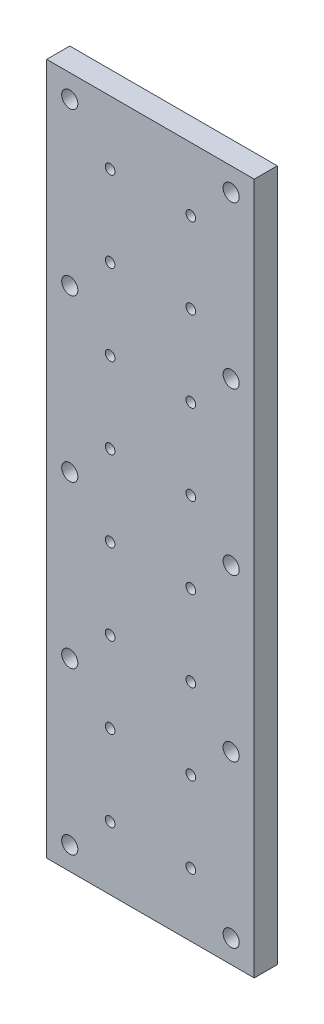
SolidWorks part; units mm, degrees
material "环氧酚醛层压布板3240"
ref_plane "Front Plane" through (0, 0, 0) normal (0, 0, 1) x (1, 0, 0)
ref_plane "Top Plane" through (0, 0, 0) normal (0, 1, 0) x (1, 0, 0)
ref_plane "Right Plane" through (0, 0, 0) normal (1, 0, 0) x (0, 0, -1)
other "Configuration Table"
sketch "Sketch1" plane through (0, 0, 0) normal (0, 0, 1) x (1, 0, 0)
  line L1 (-45, -150) -> (45, -150)
  line L2 (-45, -150) -> (-45, 150)
  line L3 (-45, 150) -> (45, 150)
  line L4 (45, -150) -> (45, 150)
  line L5 (-45, -150) -> (45, 150) construction
  line L6 (-45, 150) -> (45, -150) construction
  circle A0 centre (-35, 0) radius 5.5 construction
  point P0 (0, 0)
  dimension "D1" = 90
  dimension "D2" = 300
  dimension "D3" = 0
  dimension "D4" = 35
extrude "Boss-Extrude1" add sketch "Sketch1" along normal blind 10
hole_wizard "Ø7.0 (7) Diameter Hole1" positions "Sketch2" profile "Sketch4" hole size "Ø7.0" standard "GB" end condition through all
sketch "Sketch2" plane through (0, 0, 10) normal (0, 0, 1) x (1, 0, 0)
  point P0 (-35, 0)
sketch "Sketch4" plane through (-35, 0, 10) normal (1, 0, 0) x (0, -1, 0)
  line L0 (0, 0) -> (0, 10)
  line L1 (0, 10) -> (3.5, 10)
  line L2 (3.5, 10) -> (3.5, 0)
  line L5 (3.5, 0) -> (0, 0)
  line L11 (0, -6.35) -> (0, 107.95) construction
  dimension "通孔孔直径" = 7
  dimension "通孔孔深度" = 10
pattern_linear "LPattern1" count 3 spacing 70 along (0, -1, 0) count 2 spacing 70 along (1, 0, 0) of "Ø7.0 (7) Diameter Hole1"
pattern_linear "LPattern2" count 3 spacing 70 along (0, 1, 0) of "LPattern1", "Ø7.0 (7) Diameter Hole1"
sketch "Sketch5" plane through (0, 0, 0) normal (0, 0, -1) x (-1, 0, 0)
  line L0 (45, -150) -> (-45, 150) construction
  line L1 (-17.5, -17.5) -> (17.5, -17.5)
  line L2 (-17.5, -17.5) -> (-17.5, 17.5)
  line L3 (-17.5, 17.5) -> (17.5, 17.5)
  line L4 (17.5, -17.5) -> (17.5, 17.5)
  line L5 (-17.5, -17.5) -> (17.5, 17.5) construction
  line L6 (-17.5, 17.5) -> (17.5, -17.5) construction
  point P0 (0, 0)
  dimension "D1" = 35
  dimension "D2" = 35
hole_wizard "M5 Tapped Hole1" positions "Sketch6" profile "Sketch7" tap size "M5" standard "GB" end condition through all
sketch "Sketch6" plane through (0, 0, 0) normal (0, 0, -1) x (-1, 0, 0)
  point P0 (17.5, 17.5)
  point P3 (17.5, -17.5)
  point P6 (-17.5, -17.5)
  point P9 (-17.5, 17.5)
sketch "Sketch7" plane through (-17.5, 17.5, 0) normal (1, 0, 0) x (0, 1, 0)
  line L0 (0, 0) -> (0, 10)
  line L1 (0, 10) -> (2.1, 10)
  line L2 (2.1, 10) -> (2.1, 0)
  line L5 (2.1, 0) -> (0, 0)
  line L11 (0, -6.35) -> (0, 107.95) construction
  dimension "通孔螺纹孔钻头直径" = 4.2
  dimension "通孔螺纹孔钻头深度" = 10
cosmetic thread "Cosmetic thread 2" parameters "D2"=5
cosmetic thread "Cosmetic thread 3" parameters "D2"=5
cosmetic thread "Cosmetic thread 4" parameters "D2"=5
cosmetic thread "Cosmetic thread 5" parameters "D2"=5
pattern_linear "LPattern3" count 4 spacing 35 along (0, -1, 0) count 4 spacing 35 along (0, 1, 0) seed only of "M5 Tapped Hole1"
